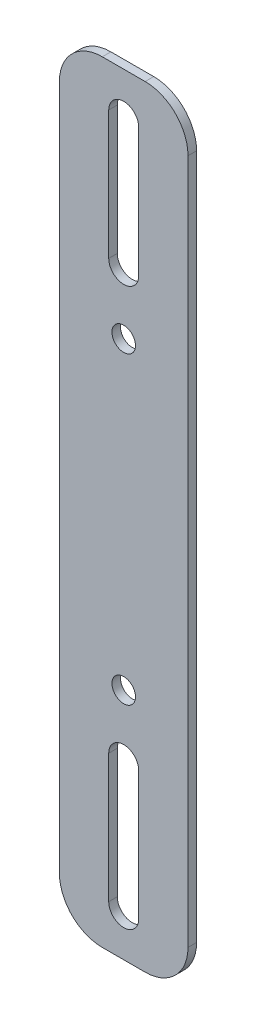
SolidWorks part; units mm, degrees
ref_plane "Front Plane" through (0, 0, 0) normal (0, 0, 1) x (1, 0, 0)
ref_plane "Top Plane" through (0, 0, 0) normal (0, 1, 0) x (1, 0, 0)
ref_plane "Right Plane" through (0, 0, 0) normal (1, 0, 0) x (0, 0, -1)
sketch "Sketch1" plane through (0, 0, 0) normal (0, 0, 1) x (1, 0, 0)
  line L1 (15, -90) -> (-15, -90)
  line L2 (15, -90) -> (15, 90)
  line L3 (15, 90) -> (-15, 90)
  line L4 (-15, -90) -> (-15, 90)
  line L5 (15, -90) -> (-15, 90) construction
  line L6 (15, 90) -> (-15, -90) construction
  point P0 (0, 0)
  dimension "D1" = 180
  dimension "D2" = 30
extrude "Boss-Extrude1" add sketch "Sketch1" along normal blind 2
fillet "Fillet1" radius 10 4 edges at (15, -90, 1) (-15, -90, 1) (-15, 90, 1) (15, 90, 1)
sketch "Sketch2" plane through (0, 0, 2) normal (0, 0, 1) x (1, 0, 0)
  line L0 (0, 80) -> (0, 50) construction
  line L1 (3.5, 80) -> (3.5, 50)
  line L2 (-3.5, 80) -> (-3.5, 50)
  arc A0 (3.5, 80) -> (-3.5, 80) centre (0, 80) ccw
  arc A1 (-3.5, 50) -> (3.5, 50) centre (0, 50) ccw
  point P3 (0, 65)
  dimension "D2" = 3.5
  dimension "D1" = 30
  dimension "D3" = 65
extrude "Cut-Extrude1" cut sketch "Sketch2" against normal through all
mirror "Mirror1" about plane through (0, 0, 0) normal (0, 1, 0) of "Cut-Extrude1"
sketch "Sketch3" plane through (0, 0, 2) normal (0, 0, 1) x (1, 0, 0)
  circle A0 centre (0, -35.5) radius 2.75
  circle A1 centre (0, 35.5) radius 2.75
  dimension "D1" = 71
  dimension "D2" = 35.5
  dimension "D3" = 5.5
extrude "Cut-Extrude2" cut sketch "Sketch3" against normal through all
sketch "Sketch4" plane through (0, 0, 2) normal (0, 0, 1) x (1, 0, 0)
  line L0 (0, 0) -> (87.5351, 0) construction
  line L1 (-15, 80) -> (-15, -80) construction
  line L2 (35, -30) -> (-15, -30)
  line L3 (35, -30) -> (35, 30)
  line L4 (35, 30) -> (-15, 30)
  line L5 (-15, -30) -> (-15, 30)
  line L6 (35, -30) -> (-15, 30) construction
  line L7 (35, 30) -> (-15, -30) construction
  point P3 (10, 0)
  dimension "D1" = 50
  dimension "D2" = 60
